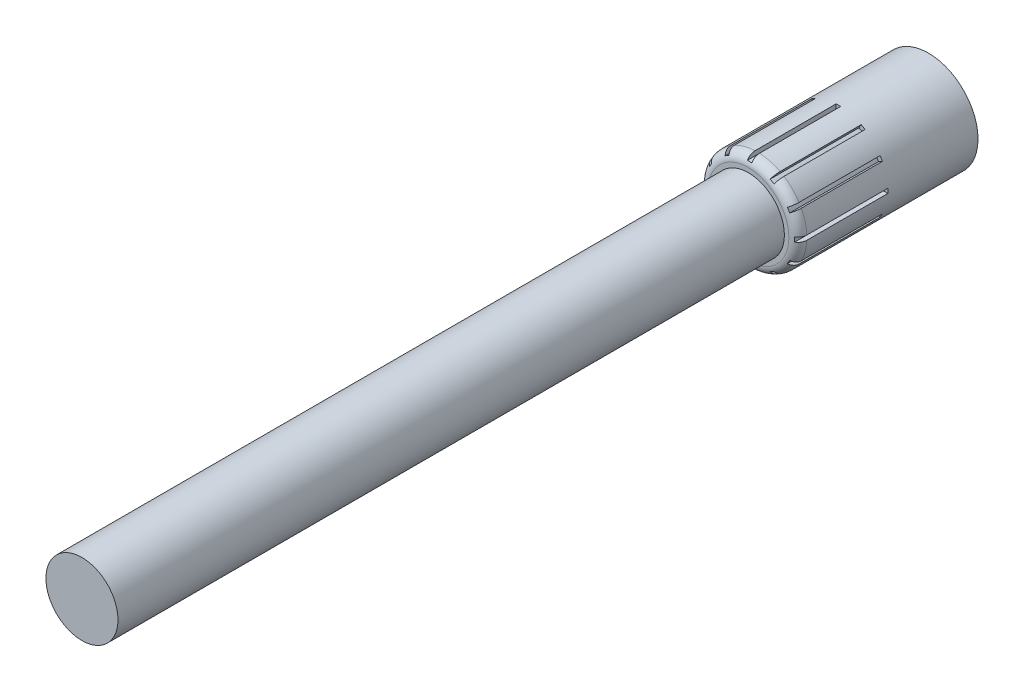
from build123d import *

# Parameters (mm, degrees)
BOSS_EXTRUDE1_DEPTH      = 100
BOSS_EXTRUDE1_DEPTH_BACK = 100
SKETCH1_R                = 55
FILLET1_R                = 10
CUT_EXTRUDE1_DEPTH       = 100
SKETCH3_R                = 40
BOSS_EXTRUDE2_DEPTH      = 740


with BuildPart() as part:
    # Sketch1 → Boss-Extrude1 (new, two sides: drawn at the far end of the back side and taken through both)
    with BuildSketch(Plane.XY.offset(-BOSS_EXTRUDE1_DEPTH_BACK)):
        with Locations((-599.884196758, -90)):
            Circle(SKETCH1_R)
    extrude(amount=BOSS_EXTRUDE1_DEPTH + BOSS_EXTRUDE1_DEPTH_BACK)

    # Fillet1
    fillet1_edges = [part.edges().sort_by_distance(p)[0] for p in [
        (-654.884196758, -90, 100),
    ]]
    fillet(fillet1_edges, radius=FILLET1_R)

    # Sketch2 → Cut-Extrude1 (cut)
    with BuildSketch(Plane.XY.offset(100)):
        with BuildLine():
            Line((-627.017990712, -131.99710973), (-629.520836487, -136.332165777))
            ThreePointArc((-629.520836487, -136.332165777), (-627.384196758, -137.631397208), (-625.190709468, -138.832165777))
            Line((-625.190709468, -138.832165777), (-622.687863693, -134.49710973))
            ThreePointArc((-622.687863693, -134.49710973), (-624.884196758, -133.301270189), (-627.017990712, -131.99710973))
        make_face()
        with BuildLine():
            ThreePointArc((-648.716362535, -115.30651271), (-647.515593966, -117.5), (-646.216362535, -119.636639729))
            Line((-646.216362535, -119.636639729), (-641.881306488, -117.133793954))
            ThreePointArc((-641.881306488, -117.133793954), (-643.185466947, -115), (-644.381306488, -112.803666935))
            Line((-644.381306488, -112.803666935), (-648.716362535, -115.30651271))
        make_face()
        with BuildLine():
            Line((-602.384196758, -139.937460889), (-602.384196758, -144.94315244))
            ThreePointArc((-602.384196758, -144.94315244), (-599.884196758, -145), (-597.384196758, -144.94315244))
            Line((-597.384196758, -144.94315244), (-597.384196758, -139.937460889))
            ThreePointArc((-597.384196758, -139.937460889), (-599.884196758, -140), (-602.384196758, -139.937460889))
        make_face()
        with BuildLine():
            ThreePointArc((-654.827349198, -87.5), (-654.884196758, -90), (-654.827349198, -92.5))
            Line((-654.827349198, -92.5), (-649.821657647, -92.5))
            ThreePointArc((-649.821657647, -92.5), (-649.884196758, -90), (-649.821657647, -87.5))
            Line((-649.821657647, -87.5), (-654.827349198, -87.5))
        make_face()
        with BuildLine():
            Line((-577.080529823, -134.49710973), (-574.577684048, -138.832165777))
            ThreePointArc((-574.577684048, -138.832165777), (-572.384196758, -137.631397208), (-570.247557029, -136.332165777))
            Line((-570.247557029, -136.332165777), (-572.750402804, -131.99710973))
            ThreePointArc((-572.750402804, -131.99710973), (-574.884196758, -133.301270189), (-577.080529823, -134.49710973))
        make_face()
        with BuildLine():
            ThreePointArc((-646.216362535, -60.363360271), (-647.515593966, -62.5), (-648.716362535, -64.69348729))
            Line((-648.716362535, -64.69348729), (-644.381306488, -67.196333065))
            ThreePointArc((-644.381306488, -67.196333065), (-643.185466947, -65), (-641.881306488, -62.866206046))
            Line((-641.881306488, -62.866206046), (-646.216362535, -60.363360271))
        make_face()
        with BuildLine():
            Line((-557.887087028, -117.133793954), (-553.552030981, -119.636639729))
            ThreePointArc((-553.552030981, -119.636639729), (-552.25279955, -117.5), (-551.052030981, -115.30651271))
            Line((-551.052030981, -115.30651271), (-555.387087028, -112.803666935))
            ThreePointArc((-555.387087028, -112.803666935), (-556.582926569, -115), (-557.887087028, -117.133793954))
        make_face()
        with BuildLine():
            ThreePointArc((-625.190709468, -41.167834223), (-627.384196758, -42.368602792), (-629.520836487, -43.667834223))
            Line((-629.520836487, -43.667834223), (-627.017990712, -48.00289027))
            ThreePointArc((-627.017990712, -48.00289027), (-624.884196758, -46.698729811), (-622.687863693, -45.50289027))
            Line((-622.687863693, -45.50289027), (-625.190709468, -41.167834223))
        make_face()
        with BuildLine():
            Line((-549.946735869, -92.5), (-544.941044318, -92.5))
            ThreePointArc((-544.941044318, -92.5), (-544.884196758, -90), (-544.941044318, -87.5))
            Line((-544.941044318, -87.5), (-549.946735869, -87.5))
            ThreePointArc((-549.946735869, -87.5), (-549.884196758, -90), (-549.946735869, -92.5))
        make_face()
        with BuildLine():
            ThreePointArc((-597.384196758, -35.05684756), (-599.884196758, -35), (-602.384196758, -35.05684756))
            Line((-602.384196758, -35.05684756), (-602.384196758, -40.062539111))
            ThreePointArc((-602.384196758, -40.062539111), (-599.884196758, -40), (-597.384196758, -40.062539111))
            Line((-597.384196758, -40.062539111), (-597.384196758, -35.05684756))
        make_face()
        with BuildLine():
            ThreePointArc((-570.247557029, -43.667834223), (-572.384196758, -42.368602792), (-574.577684048, -41.167834223))
            Line((-574.577684048, -41.167834223), (-577.080529823, -45.50289027))
            ThreePointArc((-577.080529823, -45.50289027), (-574.884196758, -46.698729811), (-572.750402804, -48.00289027))
            Line((-572.750402804, -48.00289027), (-570.247557029, -43.667834223))
        make_face()
        with BuildLine():
            Line((-555.387087028, -67.196333065), (-551.052030981, -64.69348729))
            ThreePointArc((-551.052030981, -64.69348729), (-552.25279955, -62.5), (-553.552030981, -60.363360271))
            Line((-553.552030981, -60.363360271), (-557.887087028, -62.866206046))
            ThreePointArc((-557.887087028, -62.866206046), (-556.582926569, -65), (-555.387087028, -67.196333065))
        make_face()
    extrude(amount=-CUT_EXTRUDE1_DEPTH, mode=Mode.SUBTRACT)

    # Sketch3 → Boss-Extrude2 (add)
    with BuildSketch(Plane.XY.offset(100)):
        with Locations((-599.884196758, -90)):
            Circle(SKETCH3_R)
    extrude(amount=BOSS_EXTRUDE2_DEPTH)


solid = part.part
